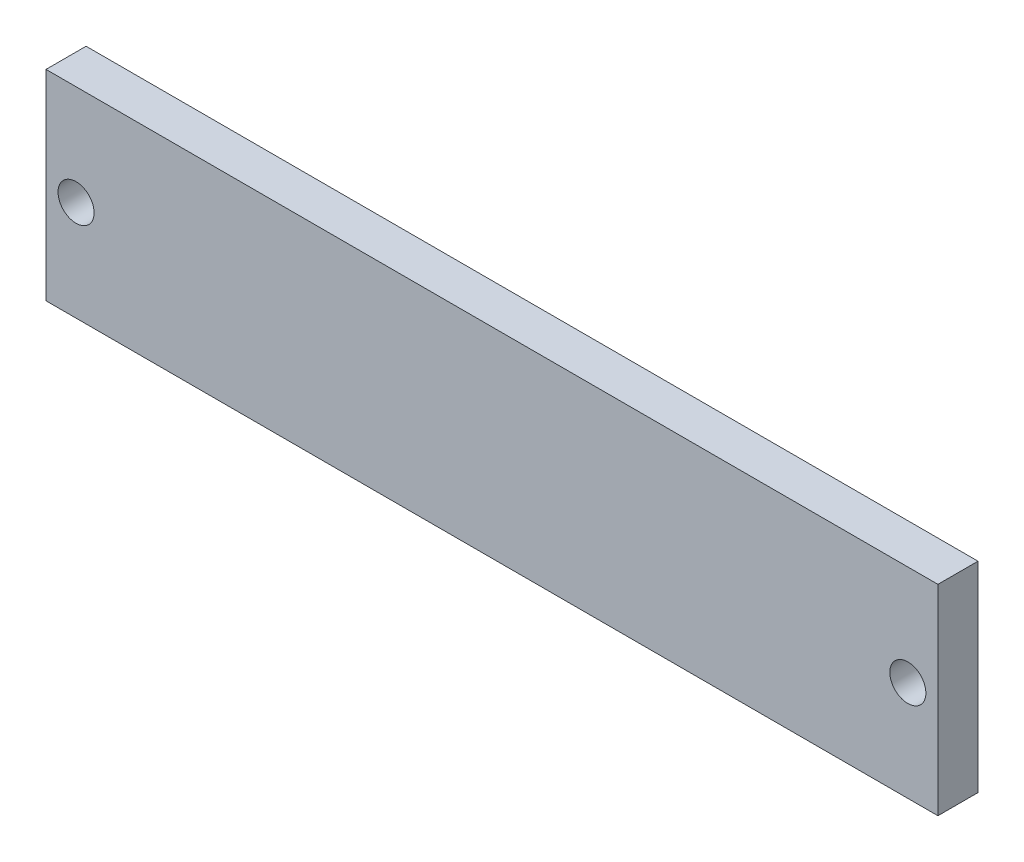
SolidWorks part; units mm, degrees
material "Q235"
ref_plane "Front Plane" through (0, 0, 0) normal (0, 0, 1) x (1, 0, 0)
ref_plane "Top Plane" through (0, 0, 0) normal (0, 1, 0) x (1, 0, 0)
ref_plane "Right Plane" through (0, 0, 0) normal (1, 0, 0) x (0, 0, -1)
sketch "Sketch1" plane through (0, 0, 0) normal (0, 0, 1) x (1, 0, 0)
  line L0 (0, 50) -> (445, 50) construction
  line L1 (0, 0) -> (445, 0)
  line L2 (0, 0) -> (0, 100)
  line L3 (0, 100) -> (445, 100)
  line L4 (445, 0) -> (445, 100)
  line L5 (222.5, 100) -> (222.5, 0) construction
  circle A0 centre (15, 50) radius 9
  circle A1 centre (430, 50) radius 9
  dimension "D3" = 18
  dimension "D4" = 415
  dimension "D1" = 445
  dimension "D2" = 100
extrude "Boss-Extrude1" add sketch "Sketch1" along normal blind 20
